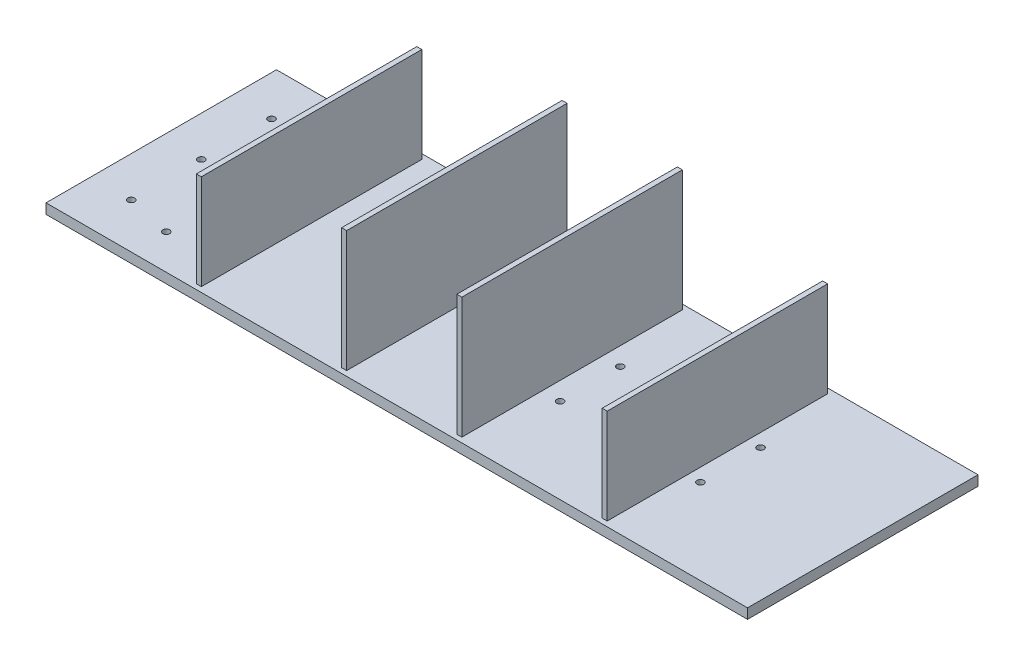
SolidWorks part; units mm, degrees
material "Q235"
ref_plane "Front Plane" through (0, 0, 0) normal (0, 0, 1) x (1, 0, 0)
ref_plane "Top Plane" through (0, 0, 0) normal (0, 1, 0) x (1, 0, 0)
ref_plane "Right Plane" through (0, 0, 0) normal (1, 0, 0) x (0, 0, -1)
sketch "Sketch1" plane through (0, 0, 0) normal (0, 1, 0) x (1, 0, 0)
  line L1 (0, 0) -> (700, 0)
  line L2 (0, 0) -> (0, -230)
  line L3 (0, -230) -> (700, -230)
  line L4 (700, 0) -> (700, -230)
  dimension "D1" = 700
  dimension "D2" = 230
extrude "Boss-Extrude1" add sketch "Sketch1" along normal blind 10
hole_wizard "M8 Tapped Hole1" positions "Sketch2" profile "Sketch3" tap size "M8" standard "GB" end condition through all
sketch "Sketch2" plane through (0, 10, 0) normal (0, 1, 0) x (1, 0, 0)
  line L0 (350, 0) -> (350, -230) construction
  line L1 (700, 0) -> (0, 0) construction
  line L2 (0, -230) -> (700, -230) construction
  line L4 (350, -115) -> (439.2488, -115) construction
  point P0 (272, -85)
  point P2 (272, -145)
  point P4 (132, -145)
  point P6 (132, -85)
  point P17 (568, -85)
  point P18 (568, -145)
  point P19 (428, -145)
  point P20 (428, -85)
  dimension "D1" = 156
  dimension "D2" = 140
  dimension "D3" = 60
sketch "Sketch3" plane through (272, 10, 85) normal (1, 0, 0) x (0, 0, 1)
  line L0 (0, 0) -> (0, 10)
  line L1 (0, 10) -> (3.4, 10)
  line L2 (3.4, 10) -> (3.4, 0)
  line L5 (3.4, 0) -> (0, 0)
  line L11 (0, -6.35) -> (0, 107.95) construction
  dimension "通孔螺纹孔钻头直径" = 6.8
  dimension "通孔螺纹孔钻头深度" = 10
cosmetic thread "Cosmetic Thread1" parameters "D2"=8
cosmetic thread "Cosmetic Thread2" parameters "D2"=8
cosmetic thread "Cosmetic Thread3" parameters "D2"=8
cosmetic thread "Cosmetic Thread4" parameters "D2"=8
cosmetic thread "Cosmetic Thread5" parameters "D2"=8
cosmetic thread "Cosmetic Thread6" parameters "D2"=8
cosmetic thread "Cosmetic Thread7" parameters "D2"=8
cosmetic thread "Cosmetic Thread8" parameters "D2"=8
hole_wizard "M8 Tapped Hole2" positions "Sketch6" profile "Sketch7" tap size "M8" standard "GB"
sketch "Sketch6" plane through (0, 10, 0) normal (0, 1, 0) x (1, 0, 0)
  line L0 (0, -100) -> (31.5112, -100) construction
  line L1 (0, 0) -> (0, -200) construction
  line L2 (350, 0) -> (350, -67.5) construction
  line L3 (700, 0) -> (0, 0) construction
  point P0 (30, -70)
  point P2 (30, -130)
  point P11 (20, -40)
  point P13 (20, -160)
  point P24 (680, -160)
  point P25 (670, -130)
  point P26 (670, -70)
  point P27 (680, -40)
  dimension "D1" = 60
  dimension "D2" = 30
  dimension "D3" = 10
  dimension "D4" = 120
sketch "Sketch7" plane through (30, 10, 70) normal (1, 0, 0) x (0, 0, 1)
  line L0 (0, 0) -> (0, 10)
  line L1 (0, 10) -> (3.4, 10)
  line L2 (3.4, 10) -> (3.4, 0)
  line L5 (3.4, 0) -> (0, 0)
  line L11 (0, -6.35) -> (0, 107.95) construction
  dimension "通孔螺纹孔钻头直径" = 6.8
  dimension "通孔螺纹孔钻头深度" = 10
cosmetic thread "Cosmetic Thread9" [suppressed] parameters "D2"=8
cosmetic thread "Cosmetic Thread10" [suppressed] parameters "D2"=8
cosmetic thread "Cosmetic Thread11" [suppressed] parameters "D2"=8
cosmetic thread "Cosmetic Thread12" [suppressed] parameters "D2"=8
cosmetic thread "Cosmetic Thread13" [suppressed] parameters "D2"=8
cosmetic thread "Cosmetic Thread14" [suppressed] parameters "D2"=8
cosmetic thread "Cosmetic Thread15" [suppressed] parameters "D2"=8
cosmetic thread "Cosmetic Thread16" [suppressed] parameters "D2"=8
sketch "Sketch8" plane through (0, 10, 0) normal (0, 1, 0) x (1, 0, 0)
  line L0 (700, 0) -> (0, 0) construction
  line L1 (290, -5) -> (295, -5)
  line L2 (290, -5) -> (290, -225)
  line L3 (290, -225) -> (295, -225)
  line L4 (295, -5) -> (295, -225)
  line L5 (0, -230) -> (700, -230) construction
  line L6 (350, 0) -> (350, -230) construction
  line L7 (405, -5) -> (405, -225)
  line L8 (410, -225) -> (405, -225)
  line L9 (410, -5) -> (410, -225)
  line L10 (410, -5) -> (405, -5)
  dimension "D1" = 5
  dimension "D2" = 110
  dimension "D3" = 5
  dimension "D4" = 5
extrude "Boss-Extrude2" add sketch "Sketch8" along normal blind 121
sketch "Sketch9" plane through (0, 10, 0) normal (0, 1, 0) x (1, 0, 0)
  line L1 (145, -5) -> (150, -5)
  line L2 (145, -5) -> (145, -225)
  line L3 (145, -225) -> (150, -225)
  line L4 (150, -5) -> (150, -225)
  line L6 (350, 0) -> (350, -230) construction
  line L7 (700, 0) -> (0, 0) construction
  line L8 (0, -230) -> (700, -230) construction
  line L9 (550, -5) -> (550, -225)
  line L10 (555, -225) -> (550, -225)
  line L11 (555, -5) -> (555, -225)
  line L12 (555, -5) -> (550, -5)
  line L13 (700, 0) -> (0, 0) construction
  line L14 (0, -230) -> (700, -230) construction
  dimension "D1" = 5
  dimension "D2" = 400
  dimension "D3" = 5
  dimension "D4" = 5
extrude "Boss-Extrude3" add sketch "Sketch9" along normal blind 95
hole_wizard "M8 Tapped Hole3" positions "Sketch10" profile "Sketch11" tap size "M8" standard "GB"
sketch "Sketch10" plane through (0, 0, 0) normal (0, -1, 0) x (-1, 0, 0)
  line L0 (0, -115) -> (-40, -115) construction
  line L1 (0, 0) -> (0, -230) construction
  point P0 (-85, -35)
  point P2 (-40, -45)
  point P4 (-40, -185)
  point P6 (-85, -195)
  point P8 (-40, -115)
  point P10 (-85, -115)
  dimension "D1" = 140
  dimension "D2" = 160
  dimension "D3" = 85
  dimension "D4" = 45
sketch "Sketch11" plane through (85, 0, 35) normal (1, 0, 0) x (0, 0, -1)
  line L0 (0, 0) -> (0, 21.7929)
  line L1 (0, 21.7929) -> (3.4, 19.75)
  line L2 (3.4, 19.75) -> (3.4, 0)
  line L5 (3.4, 0) -> (0, 0)
  line L10 (0, 21.7929) -> (-3.4, 19.75) construction
  line L11 (0, -6.35) -> (0, 107.95) construction
  dimension "螺纹孔钻头直径" = 6.8
  dimension "螺纹孔钻头深度" = 19.75
  dimension "导头角度" = 118
cosmetic thread "Cosmetic Thread17" parameters "D1"=10, "D2"=8
cosmetic thread "Cosmetic Thread18" parameters "D1"=10, "D2"=8
cosmetic thread "Cosmetic Thread19" parameters "D1"=10, "D2"=8
cosmetic thread "Cosmetic Thread20" parameters "D1"=10, "D2"=8
cosmetic thread "Cosmetic Thread21" parameters "D1"=10, "D2"=8
cosmetic thread "Cosmetic Thread22" parameters "D1"=10, "D2"=8
